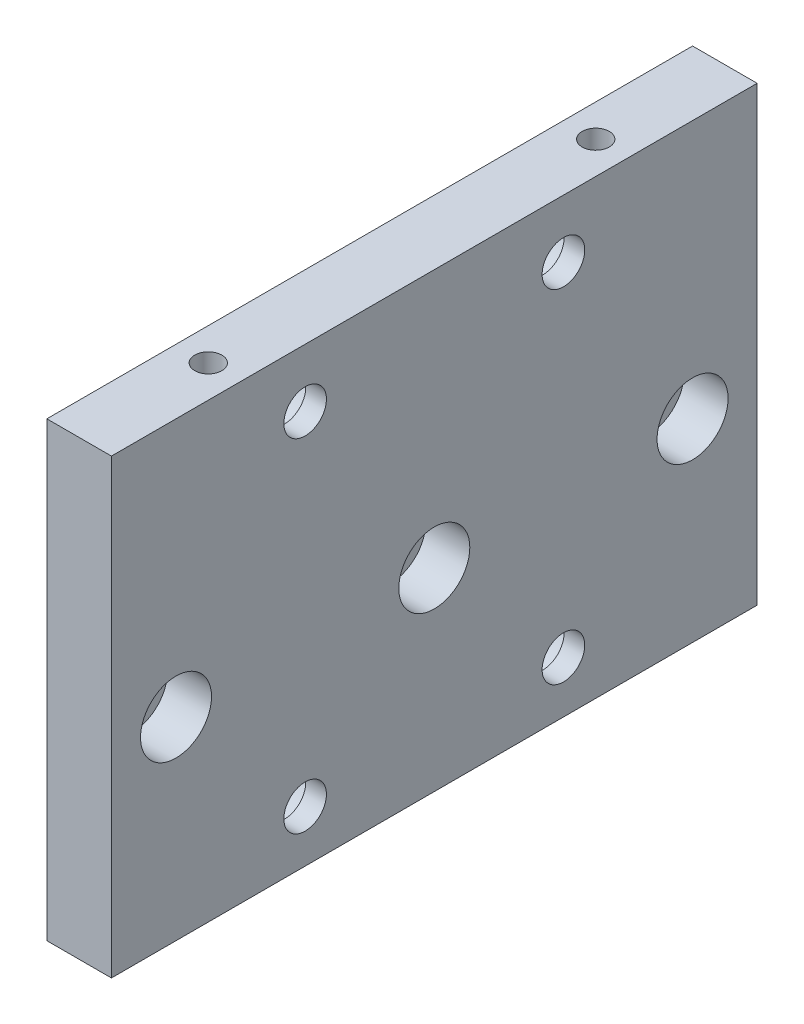
from build123d import *

# Parameters (mm, degrees)
SKETCH_1_W                = 100
SKETCH_1_H                = 70
EXTRUDE_1_DEPTH           = 10
HOLE_WIZARD_1_D           = 6.6
HOLE_WIZARD_1_DEPTH       = 15
HOLE_WIZARD_1_CBORE_D     = 11
HOLE_WIZARD_1_CBORE_DEPTH = 6.8
HOLE_WIZARD_1_TIP         = 1.982840043
HOLE_WIZARD_3_AT_2_COUNT  = 2
HOLE_WIZARD_3_AT_2_PITCH  = 40
HOLE_WIZARD_3_AT_3_COUNT  = 2
HOLE_WIZARD_3_AT_3_PITCH  = 53
HOLE_WIZARD_3_AT_4_COUNT  = 2
HOLE_WIZARD_3_AT_4_PITCH  = 66.400301204
HOLE_WIZARD_M5_1_D        = 4.2
HOLE_WIZARD_M5_1_DEPTH    = 12.4
HOLE_WIZARD_M5_1_TIP      = 1.2618073


with BuildPart() as part:
    # 草图1 → 凸台-拉伸1 (new body)
    with BuildSketch(Plane(origin=(0, 0, 0), x_dir=(0, 0, -1), z_dir=(1, 0, 0))):
        Rectangle(SKETCH_1_W, SKETCH_1_H)
    extrude(amount=EXTRUDE_1_DEPTH)

    # 打孔尺寸(%根据)内六角圆柱头螺钉的类型1
    with Locations(Plane(origin=(10, 0, 0), x_dir=(0, 0, -1), z_dir=(1, 0, 0))):
        with Locations((-40, -5), (0, -5), (40, -5)):
            CounterBoreHole(HOLE_WIZARD_1_D / 2, HOLE_WIZARD_1_CBORE_D / 2, HOLE_WIZARD_1_CBORE_DEPTH, depth=HOLE_WIZARD_1_DEPTH)
            with Locations((0, 0, -(HOLE_WIZARD_1_DEPTH + HOLE_WIZARD_1_TIP / 2))):  # 118° drill point
                Cone(0, HOLE_WIZARD_1_D / 2, HOLE_WIZARD_1_TIP, mode=Mode.SUBTRACT)

    # 草图9 → 打孔尺寸(%根据)内六角圆柱头螺钉的类型3 (revolve, cut)
    with BuildSketch(Plane(origin=(0, 26, -20), x_dir=(0, 0, 1), z_dir=(0, 1, 0))):
        Polygon((0, 0), (0, 10), (3.3, 10), (3.3, 6.8), (5.5, 6.8), (5.5, 0.025), (5.525, 0), align=None)
    hole_wizard_3 = revolve(axis=Axis((-6.35, 26, -20), (1, 0, 0)), mode=Mode.SUBTRACT)

    # 打孔尺寸(%根据)内六角圆柱头螺钉的类型3 at 2: 打孔尺寸(%根据)内六角圆柱头螺钉的类型3 ×2
    with Locations(*[(0, 0, i * HOLE_WIZARD_3_AT_2_PITCH) for i in range(1, HOLE_WIZARD_3_AT_2_COUNT)]):
        add(hole_wizard_3, mode=Mode.SUBTRACT)

    # 打孔尺寸(%根据)内六角圆柱头螺钉的类型3 at 3: 打孔尺寸(%根据)内六角圆柱头螺钉的类型3 ×2
    with Locations(*[(0, -i * HOLE_WIZARD_3_AT_3_PITCH, 0) for i in range(1, HOLE_WIZARD_3_AT_3_COUNT)]):
        add(hole_wizard_3, mode=Mode.SUBTRACT)

    # 打孔尺寸(%根据)内六角圆柱头螺钉的类型3 at 4: 打孔尺寸(%根据)内六角圆柱头螺钉的类型3 ×2
    with Locations(*[Vector(0, -0.7981891503332307, 0.6024069059118724) * (i * HOLE_WIZARD_3_AT_4_PITCH) for i in range(1, HOLE_WIZARD_3_AT_4_COUNT)]):
        add(hole_wizard_3, mode=Mode.SUBTRACT)

    # M5 螺纹孔1
    with Locations(Plane(origin=(0, 35, 0), x_dir=(1, 0, 0), z_dir=(0, 1, 0))):
        with Locations((5, 30), (5, -30)):
            Hole(HOLE_WIZARD_M5_1_D / 2, depth=HOLE_WIZARD_M5_1_DEPTH)
            with Locations((0, 0, -(HOLE_WIZARD_M5_1_DEPTH + HOLE_WIZARD_M5_1_TIP / 2))):  # 118° drill point
                Cone(0, HOLE_WIZARD_M5_1_D / 2, HOLE_WIZARD_M5_1_TIP, mode=Mode.SUBTRACT)


solid = part.part
